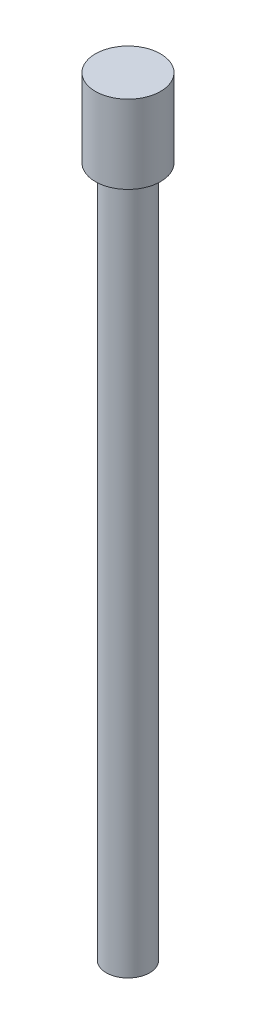
SolidWorks part; units mm, degrees
material "Q235B"
ref_plane "Front Plane" through (0, 0, 0) normal (0, 0, 1) x (1, 0, 0)
ref_plane "Top Plane" through (0, 0, 0) normal (0, 1, 0) x (1, 0, 0)
ref_plane "Right Plane" through (0, 0, 0) normal (1, 0, 0) x (0, 0, -1)
sketch "Sketch1" plane through (0, 0, 0) normal (0, 0, 1) x (1, 0, 0)
  line L0 (0, 0) -> (20, 0)
  line L1 (20, 0) -> (20, 636)
  line L2 (20, 636) -> (30, 636)
  line L3 (30, 636) -> (30, 708)
  line L4 (30, 708) -> (0, 708)
  line L5 (0, 708) -> (0, 0)
  line L6 (0, 0) -> (0, -26.2624) construction
  dimension "D1" = 40
  dimension "D2" = 60
  dimension "D3" = 72
  dimension "D4" = 708
revolve "Revolve1" add sketch "Sketch1" angle 360 about L6
